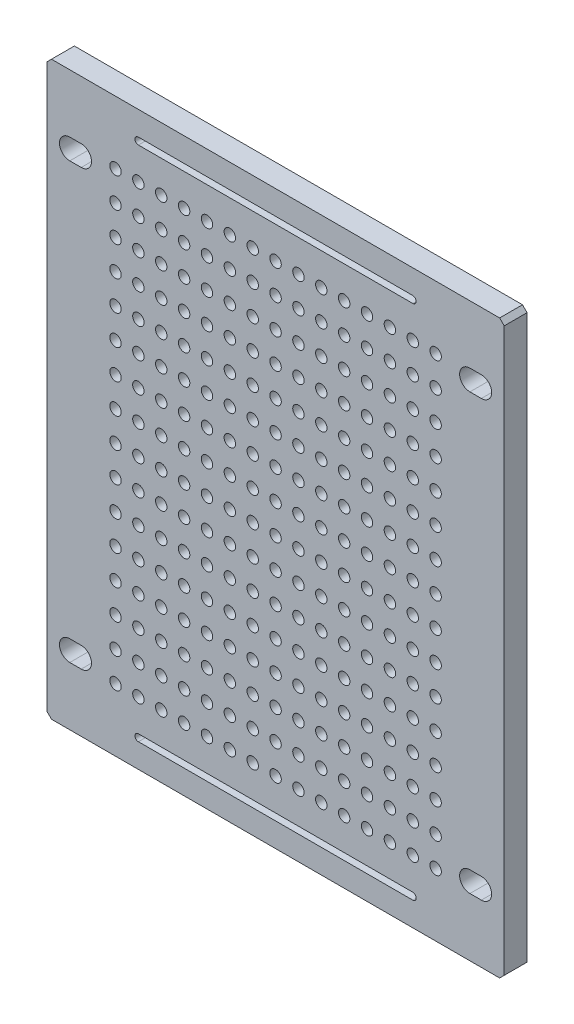
SolidWorks part; units mm, degrees
material "PE"
ref_plane "Front Plane" through (0, 0, 0) normal (0, 0, 1) x (1, 0, 0)
ref_plane "Top Plane" through (0, 0, 0) normal (0, 1, 0) x (1, 0, 0)
ref_plane "Right Plane" through (0, 0, 0) normal (1, 0, 0) x (0, 0, -1)
sketch "Sketch1" plane through (0, 0, 0) normal (0, 0, 1) x (1, 0, 0)
  line L1 (-100, 125) -> (100, 125)
  line L2 (-100, 125) -> (-100, -125)
  line L3 (-100, -125) -> (100, -125)
  line L4 (100, 125) -> (100, -125)
  line L5 (-100, 125) -> (100, -125) construction
  line L6 (-100, -125) -> (100, 125) construction
  point P0 (0, 0)
  dimension "D1" = 200
  dimension "D2" = 250
extrude "Boss-Extrude1" add sketch "Sketch1" along normal blind 10
sketch "Sketch3" plane through (0, 0, 10) normal (0, 0, 1) x (1, 0, 0)
  line L0 (100, 125) -> (-100, 125) construction
  line L1 (-100, 125) -> (-100, -125) construction
  circle A0 centre (-70, 97.5) radius 2.5
  dimension "D1" = 5
  dimension "D2" = 27.5
  dimension "D3" = 30
extrude "Cut-Extrude1" cut sketch "Sketch3" against normal through all
pattern_linear "LPattern1" count 15 spacing 10 along (1, 0, 0) of "Cut-Extrude1"
pattern_linear "LPattern2" count 16 spacing 13 along (0, -1, 0) of "LPattern1", "Cut-Extrude1"
pattern_linear "LPattern3" [suppressed] count 2 spacing 260
sketch "Sketch5" plane through (0, 0, 10) normal (0, 0, 1) x (1, 0, 0)
  line L0 (-60, 113) -> (60, 113) construction
  line L1 (-60, 114.5) -> (60, 114.5)
  line L2 (-60, 111.5) -> (60, 111.5)
  line L4 (0, 125) -> (0, -43.963) construction
  line L7 (100, 125) -> (-100, 125) construction
  line L10 (-100, 0) -> (-134.7946, 0) construction
  line L11 (-100, 125) -> (-100, -125) construction
  line L15 (-60, -113) -> (60, -113) construction
  line L16 (-60, -114.5) -> (60, -114.5)
  line L17 (-60, -111.5) -> (60, -111.5)
  arc A0 (-60, 114.5) -> (-60, 111.5) centre (-60, 113) ccw
  arc A1 (60, 111.5) -> (60, 114.5) centre (60, 113) ccw
  arc A6 (-60, -114.5) -> (-60, -111.5) centre (-60, -113) cw
  arc A7 (60, -111.5) -> (60, -114.5) centre (60, -113) cw
  point P2 (0, 113)
  point P34 (0, -113)
  dimension "D3" = 12
  dimension "D1" = 3
  dimension "D2" = 120
extrude "Cut-Extrude2" cut sketch "Sketch5" against normal through all
sketch "Sketch6" plane through (0, 0, 10) normal (0, 0, 1) x (1, 0, 0)
  line L0 (-90, 95) -> (-85, 95) construction
  line L3 (-100, 0) -> (-95.4646, 0) construction
  line L4 (-100, 125) -> (-100, -125) construction
  line L5 (-90, 99.5) -> (-85, 99.5)
  line L8 (0, 125) -> (0, 86.1674) construction
  line L9 (100, 125) -> (-100, 125) construction
  line L10 (-90, 90.5) -> (-85, 90.5)
  line L13 (-90, -95) -> (-85, -95) construction
  line L16 (-90, -99.5) -> (-85, -99.5)
  line L17 (-90, -90.5) -> (-85, -90.5)
  line L18 (90, -95) -> (85, -95) construction
  line L19 (90, -99.5) -> (85, -99.5)
  line L20 (90, -90.5) -> (85, -90.5)
  line L21 (90, 95) -> (85, 95) construction
  line L22 (90, 99.5) -> (85, 99.5)
  line L23 (90, 90.5) -> (85, 90.5)
  arc A8 (-90, 99.5) -> (-90, 90.5) centre (-90, 95) ccw
  arc A9 (-85, 90.5) -> (-85, 99.5) centre (-85, 95) ccw
  arc A10 (-90, -99.5) -> (-90, -90.5) centre (-90, -95) cw
  arc A11 (-85, -90.5) -> (-85, -99.5) centre (-85, -95) cw
  arc A12 (90, -99.5) -> (90, -90.5) centre (90, -95) ccw
  arc A13 (85, -90.5) -> (85, -99.5) centre (85, -95) ccw
  arc A14 (90, 99.5) -> (90, 90.5) centre (90, 95) cw
  arc A15 (85, 90.5) -> (85, 99.5) centre (85, 95) cw
  point P2 (-87.5, 95)
  point P14 (-87.5, -95)
  point P25 (87.5, -95)
  point P32 (87.5, 95)
  dimension "D3" = 175
  dimension "D4" = 190
  dimension "D1" = 9
  dimension "D2" = 5
extrude "Cut-Extrude3" cut sketch "Sketch6" against normal blind 10
chamfer "Chamfer1" distance 2 angle 45 4 edges at (-100, -125, 5) (100, -125, 5) (100, 125, 5) (-100, 125, 5)
